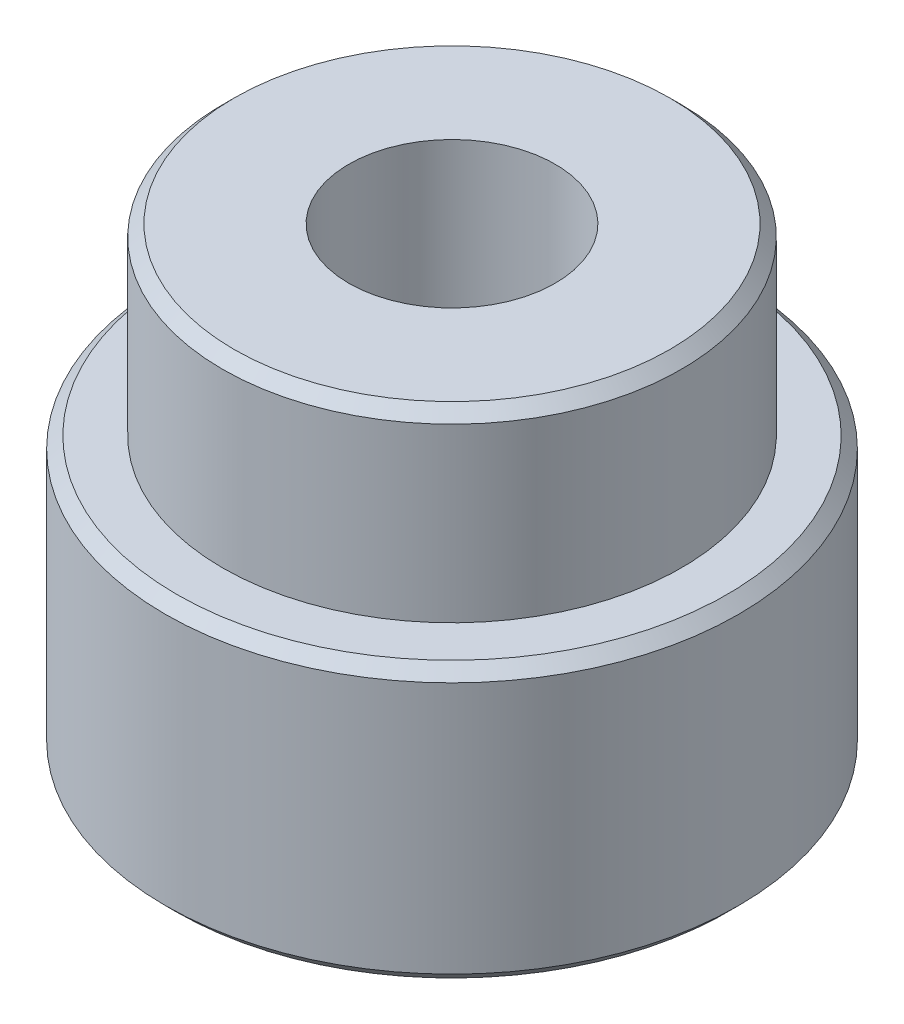
SolidWorks part; units mm, degrees
ref_plane "前视基准面" through (0, 0, 0) normal (0, 0, 1) x (1, 0, 0)
ref_plane "上视基准面" through (0, 0, 0) normal (0, 1, 0) x (1, 0, 0)
ref_plane "右视基准面" through (0, 0, 0) normal (1, 0, 0) x (0, 0, -1)
sketch "草图1" plane through (0, 0, 0) normal (0, 1, 0) x (1, 0, 0)
  circle A0 centre (0, 0) radius 10
  dimension "D1" = 20
extrude "凸台-拉伸1" add sketch "草图1" along normal blind 20
chamfer "倒角1" [suppressed] distance 0.5 angle 45
sketch "草图3" plane through (0, 0, 0) normal (0, -1, 0) x (-1, 0, 0)
  circle A0 centre (0, 0) radius 12.5
  dimension "D1" = 25
extrude "凸台-拉伸2" add sketch "草图3" against normal blind 12
sketch "草图2" plane through (0, 20, 0) normal (0, 1, 0) x (1, 0, 0)
  circle A0 centre (0, 0) radius 4.5
  dimension "D1" = 9
extrude "切除-拉伸1" cut sketch "草图2" against normal through all
chamfer "倒角2" distance 0.5 angle 45 3 edges at (0, 12, -12.5) (0, 0, -12.5) (0, 20, 10)
